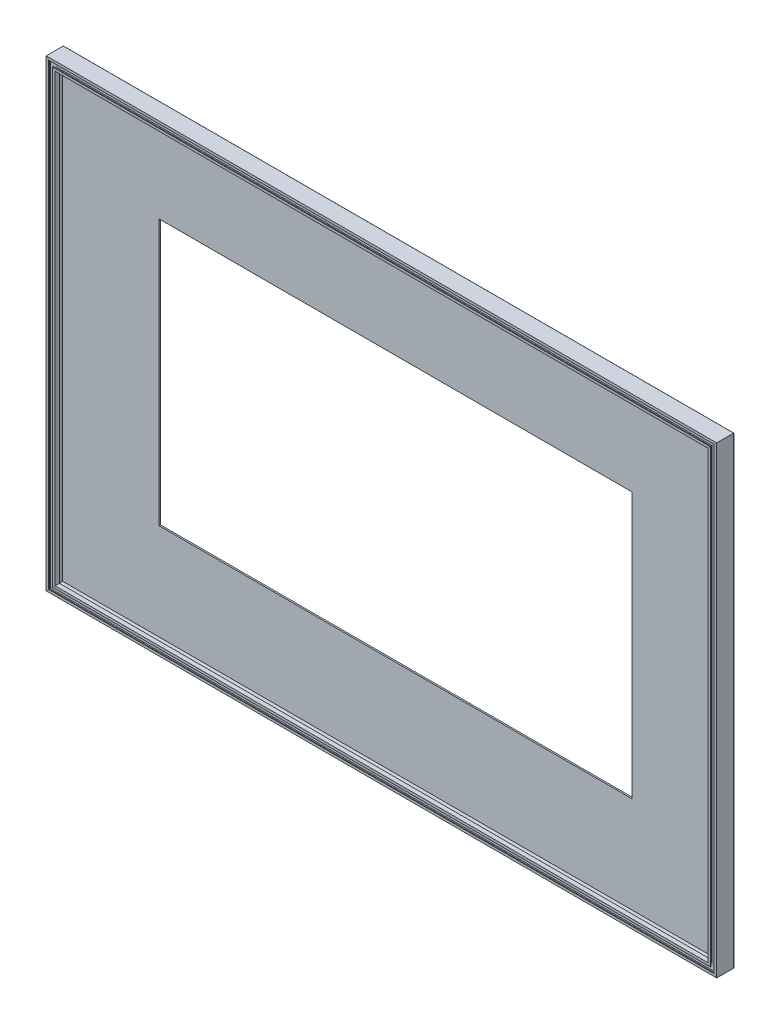
from build123d import *

# Parameters (mm, degrees)
MEMBER_1_DEPTH      = 40.357337308
MEMBER_1_DEPTH_BACK = 1400.357337308
MEMBER_1_2_DEPTH    = 1020.714674617
MEMBER_1_3_DEPTH    = 1440.714674617
MEMBER_1_4_DEPTH    = 1020.714674617
SKETCH_12_W         = 1350
SKETCH_12_H         = 930
EXTRUDE_1_DEPTH     = 3
SKETCH_13_W         = 959
SKETCH_13_H         = 539
CUT_EXTRUDE_1_DEPTH = 10


with BuildPart() as part:
    # 草图11 → Member 1 (new, two sides: drawn at the far end of the back side and taken through both)
    with BuildSketch(Plane(origin=(-680, 470, 0), x_dir=(0, -1, 0), z_dir=(-1, 0, 0)).offset(-MEMBER_1_DEPTH_BACK)):
        with BuildLine():
            Line((13, -1.5), (13, 0))
            Line((13, 0), (18, 0))
            Line((18, 0), (18, -8.7))
            Line((18, -8.7), (2, -8.7))
            Line((2, -8.7), (2, -32))
            ThreePointArc((2, -32), (2.292893219, -32.707106781), (3, -33))
            Line((3, -33), (8, -33))
            Line((8, -33), (8, -31.5))
            Line((8, -31.5), (10, -31.5))
            Line((10, -31.5), (10, -35))
            Line((10, -35), (0.5, -35))
            ThreePointArc((0.5, -35), (0.146446609, -34.853553391), (0, -34.5))
            Line((0, -34.5), (0, 0))
            Line((0, 0), (5, 0))
            Line((5, 0), (5, -1.5))
            Line((5, -1.5), (2, -1.5))
            Line((2, -1.5), (2, -6.7))
            Line((2, -6.7), (16, -6.7))
            Line((16, -6.7), (16, -1.5))
            Line((16, -1.5), (13, -1.5))
        make_face()
    extrude(amount=MEMBER_1_DEPTH + MEMBER_1_DEPTH_BACK)

    # Member 1 mitre 1
    split(bisect_by=Plane(origin=(-680, 470, 0), x_dir=(-0.707106781, 0.707106781, 0), z_dir=(0.707106781, 0.707106781, 0)), keep=Keep.TOP)

    # Member 1 mitre 2
    split(bisect_by=Plane(origin=(680, 470, 0), x_dir=(-0.707106781, -0.707106781, 0), z_dir=(-0.707106781, 0.707106781, 0)), keep=Keep.TOP)


with BuildPart() as body_2:
    # 草图11 on segment 2 (carried to segment 2) → Member 1 2 (new body)
    with BuildSketch(Plane(origin=(680, -510.357337308, 0), x_dir=(-1, 0, 0), z_dir=(0, 1, 0))):
        with BuildLine():
            Line((13, -1.5), (13, 0))
            Line((13, 0), (18, 0))
            Line((18, 0), (18, -8.7))
            Line((18, -8.7), (2, -8.7))
            Line((2, -8.7), (2, -32))
            ThreePointArc((2, -32), (2.292893219, -32.707106781), (3, -33))
            Line((3, -33), (8, -33))
            Line((8, -33), (8, -31.5))
            Line((8, -31.5), (10, -31.5))
            Line((10, -31.5), (10, -35))
            Line((10, -35), (0.5, -35))
            ThreePointArc((0.5, -35), (0.146446609, -34.853553391), (0, -34.5))
            Line((0, -34.5), (0, 0))
            Line((0, 0), (5, 0))
            Line((5, 0), (5, -1.5))
            Line((5, -1.5), (2, -1.5))
            Line((2, -1.5), (2, -6.7))
            Line((2, -6.7), (16, -6.7))
            Line((16, -6.7), (16, -1.5))
            Line((16, -1.5), (13, -1.5))
        make_face()
    extrude(amount=MEMBER_1_2_DEPTH)

    # Member 1 2 mitre 1
    split(bisect_by=Plane(origin=(680, 470, 0), x_dir=(0.707106781, 0.707106781, 0), z_dir=(0.707106781, -0.707106781, 0)), keep=Keep.TOP)

    # Member 1 2 mitre 2
    split(bisect_by=Plane(origin=(680, -470, 0), x_dir=(-0.707106781, 0.707106781, 0), z_dir=(0.707106781, 0.707106781, 0)), keep=Keep.TOP)


with BuildPart() as body_3:
    # 草图11 on segment 3 (carried to segment 3) → Member 1 3 (new body)
    with BuildSketch(Plane(origin=(-720.357337308, -470, 0), x_dir=(0, 1, 0), z_dir=(1, 0, 0))):
        with BuildLine():
            Line((13, -1.5), (13, 0))
            Line((13, 0), (18, 0))
            Line((18, 0), (18, -8.7))
            Line((18, -8.7), (2, -8.7))
            Line((2, -8.7), (2, -32))
            ThreePointArc((2, -32), (2.292893219, -32.707106781), (3, -33))
            Line((3, -33), (8, -33))
            Line((8, -33), (8, -31.5))
            Line((8, -31.5), (10, -31.5))
            Line((10, -31.5), (10, -35))
            Line((10, -35), (0.5, -35))
            ThreePointArc((0.5, -35), (0.146446609, -34.853553391), (0, -34.5))
            Line((0, -34.5), (0, 0))
            Line((0, 0), (5, 0))
            Line((5, 0), (5, -1.5))
            Line((5, -1.5), (2, -1.5))
            Line((2, -1.5), (2, -6.7))
            Line((2, -6.7), (16, -6.7))
            Line((16, -6.7), (16, -1.5))
            Line((16, -1.5), (13, -1.5))
        make_face()
    extrude(amount=MEMBER_1_3_DEPTH)

    # Member 1 3 mitre 1
    split(bisect_by=Plane(origin=(-680, -470, 0), x_dir=(0.707106781, 0.707106781, 0), z_dir=(0.707106781, -0.707106781, 0)), keep=Keep.TOP)

    # Member 1 3 mitre 2
    split(bisect_by=Plane(origin=(680, -470, 0), x_dir=(0.707106781, -0.707106781, 0), z_dir=(-0.707106781, -0.707106781, 0)), keep=Keep.TOP)


with BuildPart() as body_4:
    # 草图11 on segment 4 (carried to segment 4) → Member 1 4 (new body)
    with BuildSketch(Plane(origin=(-680, 510.357337308, 0), x_dir=(1, 0, 0), z_dir=(0, -1, 0))):
        with BuildLine():
            Line((13, -1.5), (13, 0))
            Line((13, 0), (18, 0))
            Line((18, 0), (18, -8.7))
            Line((18, -8.7), (2, -8.7))
            Line((2, -8.7), (2, -32))
            ThreePointArc((2, -32), (2.292893219, -32.707106781), (3, -33))
            Line((3, -33), (8, -33))
            Line((8, -33), (8, -31.5))
            Line((8, -31.5), (10, -31.5))
            Line((10, -31.5), (10, -35))
            Line((10, -35), (0.5, -35))
            ThreePointArc((0.5, -35), (0.146446609, -34.853553391), (0, -34.5))
            Line((0, -34.5), (0, 0))
            Line((0, 0), (5, 0))
            Line((5, 0), (5, -1.5))
            Line((5, -1.5), (2, -1.5))
            Line((2, -1.5), (2, -6.7))
            Line((2, -6.7), (16, -6.7))
            Line((16, -6.7), (16, -1.5))
            Line((16, -1.5), (13, -1.5))
        make_face()
    extrude(amount=MEMBER_1_4_DEPTH)

    # Member 1 4 mitre 1
    split(bisect_by=Plane(origin=(-680, 470, 0), x_dir=(0.707106781, -0.707106781, 0), z_dir=(-0.707106781, -0.707106781, 0)), keep=Keep.TOP)

    # Member 1 4 mitre 2
    split(bisect_by=Plane(origin=(-680, -470, 0), x_dir=(-0.707106781, -0.707106781, 0), z_dir=(-0.707106781, 0.707106781, 0)), keep=Keep.TOP)


with BuildPart() as body_5:
    # 草图12 → 凸台-拉伸1 (new body)
    with BuildSketch(Plane.XY.offset(-31.5)):
        Rectangle(SKETCH_12_W, SKETCH_12_H)
    extrude(amount=EXTRUDE_1_DEPTH)

    # 草图13 → 切除-拉伸1 (cut)
    with BuildSketch(Plane(origin=(0, 0, -31.5), x_dir=(-1, 0, 0), z_dir=(0, 0, -1))):
        Rectangle(SKETCH_13_W, SKETCH_13_H)
    extrude(amount=-CUT_EXTRUDE_1_DEPTH, mode=Mode.SUBTRACT)


solid = Compound([part.part, body_2.part, body_3.part, body_4.part, body_5.part])
